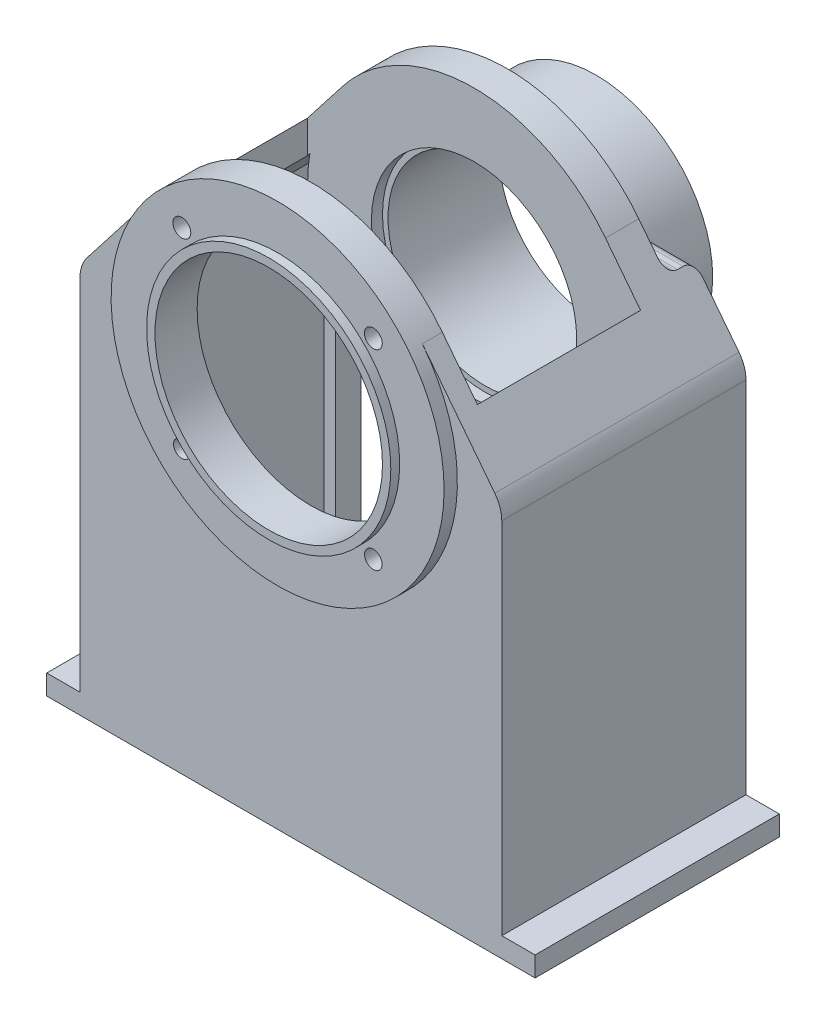
SolidWorks part; units mm, degrees
ref_plane "Front Plane" through (0, 0, 0) normal (0, 0, 1) x (1, 0, 0)
ref_plane "Top Plane" through (0, 0, 0) normal (0, 1, 0) x (1, 0, 0)
ref_plane "Right Plane" through (0, 0, 0) normal (1, 0, 0) x (0, 0, -1)
ref_plane "Plane1" through (0, 0, -1277.693) normal (0, 0, 1) x (1, 0, 0)
sketch "Sketch1" plane through (0, 0, -1277.693) normal (0, 0, 1) x (1, 0, 0)
  line L0 (671.2306, 234.744) -> (711.2306, 234.744)
  line L1 (711.2306, 234.744) -> (521.2306, 479.1294)
  line L2 (521.2306, 479.1294) -> (331.2306, 234.744)
  line L3 (331.2306, 234.744) -> (371.2306, 234.744)
  arc A0 (371.2306, 234.744) -> (671.2306, 234.744) centre (521.2306, 234.744) ccw
  dimension "D1" = 150
  dimension "D2" = 190
  dimension "D3" = 380
  dimension "D4" = 244.3855
extrude "Boss-Extrude1" add sketch "Sketch1" against normal blind 7
sketch "Sketch2" plane through (0, 234.744, 0) normal (0, -1, 0) x (1, 0, 0)
  line L0 (741.2306, -1284.693) -> (693.2306, -1284.693)
  line L1 (693.2306, -1284.693) -> (693.2306, -1277.693)
  line L2 (693.2306, -1277.693) -> (741.2306, -1277.693)
  line L3 (741.2306, -1277.693) -> (741.2306, -1284.693)
  line L4 (671.2306, -1284.693) -> (671.2306, -1277.693) construction
  line L5 (671.2306, -1277.693) -> (711.2306, -1277.693) construction
  dimension "D1" = 22
  dimension "D2" = 70
  dimension "D3" = 7
extrude "Boss-Extrude2" add sketch "Sketch2" along normal blind 352
sketch "Sketch3" plane through (0, 234.744, 0) normal (0, -1, 0) x (1, 0, 0)
  line L0 (349.2306, -1284.693) -> (331.2306, -1284.693)
  line L1 (331.2306, -1284.693) -> (331.2306, -1277.693)
  line L2 (331.2306, -1277.693) -> (349.2306, -1277.693)
  line L3 (349.2306, -1277.693) -> (349.2306, -1284.693)
  line L4 (331.2306, -1284.693) -> (331.2306, -1277.693) construction
  line L5 (331.2306, -1277.693) -> (371.2306, -1277.693) construction
  dimension "D1" = 18
  dimension "D2" = 7
extrude "Boss-Extrude3" add sketch "Sketch3" along normal blind 352
sketch "Sketch4" plane through (0, 0, -1284.693) normal (0, 0, -1) x (-1, 0, 0)
  line L0 (-331.2306, -117.256) -> (-741.2306, -117.256)
  line L1 (-741.2306, -117.256) -> (-741.2306, 234.744)
  line L2 (-741.2306, 234.744) -> (-711.2306, 234.744)
  line L3 (-711.2306, 234.744) -> (-521.2306, 479.1294)
  line L4 (-521.2306, 479.1294) -> (-331.2306, 234.744)
  line L5 (-331.2306, 234.744) -> (-331.2306, -117.256)
  line L6 (-331.2306, -117.256) -> (-331.2306, 234.744) construction
  line L7 (-331.2306, -117.256) -> (-349.2306, -117.256) construction
  dimension "D1" = 190
  dimension "D2" = 380
  dimension "D3" = 410
  dimension "D4" = 352
  dimension "D5" = 596.3855
extrude "Boss-Extrude4" add sketch "Sketch4" along normal blind 18
sketch "Sketch5" plane through (0, 0, -1277.693) normal (0, 0, 1) x (1, 0, 0)
  line L0 (371.2306, 234.744) -> (354.0306, 234.744)
  line L1 (354.0306, 234.744) -> (349.2306, 228.57)
  line L2 (349.2306, 228.57) -> (349.2306, -117.256)
  line L3 (349.2306, -117.256) -> (331.2306, -117.256)
  line L4 (331.2306, -117.256) -> (331.2306, 234.744)
  line L5 (331.2306, 234.744) -> (521.2306, 479.1294)
  line L6 (521.2306, 479.1294) -> (711.2306, 234.744)
  line L7 (711.2306, 234.744) -> (741.2306, 234.744)
  line L8 (741.2306, 234.744) -> (741.2306, -117.256)
  line L9 (741.2306, -117.256) -> (693.2306, -117.256)
  line L10 (693.2306, -117.256) -> (693.2306, 228.57)
  line L11 (693.2306, 228.57) -> (688.4306, 234.744)
  line L12 (688.4306, 234.744) -> (671.2306, 234.744)
  line L13 (741.2306, -117.256) -> (741.2306, 234.744) construction
  line L14 (741.2306, -117.256) -> (693.2306, -117.256) construction
  arc A0 (671.2306, 234.744) -> (371.2306, 234.744) centre (521.2306, 234.744) cw
  dimension "D1" = 150
  dimension "D2" = 30
  dimension "D3" = 48
  dimension "D4" = 52.8
  dimension "D5" = 220
  dimension "D6" = 387.2
  dimension "D7" = 392
  dimension "D8" = 410
  dimension "D9" = 345.8261
  dimension "D10" = 352
  dimension "D11" = 596.3855
extrude "Boss-Extrude5" add sketch "Sketch5" along normal blind 30
sketch "Sketch6" plane through (0, 0, -1247.693) normal (0, 0, 1) x (1, 0, 0)
  line L0 (371.2306, 256.8673) -> (349.2306, 228.57)
  line L1 (349.2306, 228.57) -> (349.2306, -117.256)
  line L2 (349.2306, -117.256) -> (331.2306, -117.256)
  line L3 (331.2306, -117.256) -> (331.2306, 234.744)
  line L4 (331.2306, 234.744) -> (371.2306, 286.1935)
  line L5 (371.2306, 286.1935) -> (371.2306, 256.8673)
  line L6 (741.2306, -117.256) -> (741.2306, 234.744) construction
  line L7 (693.2306, -117.256) -> (741.2306, -117.256) construction
  dimension "D1" = 370
  dimension "D2" = 392
  dimension "D3" = 410
  dimension "D4" = 345.8261
  dimension "D5" = 352
  dimension "D6" = 374.1233
  dimension "D7" = 403.4496
extrude "Boss-Extrude6" add sketch "Sketch6" along normal blind 147
sketch "Sketch7" plane through (0, 0, -1247.693) normal (0, 0, 1) x (1, 0, 0)
  line L0 (741.2306, -117.256) -> (693.2306, -117.256)
  line L1 (693.2306, -117.256) -> (693.2306, 228.57)
  line L2 (693.2306, 228.57) -> (671.2306, 256.8673)
  line L3 (671.2306, 256.8673) -> (671.2306, 286.1935)
  line L4 (671.2306, 286.1935) -> (711.2306, 234.744)
  line L5 (711.2306, 234.744) -> (741.2306, 234.744)
  line L6 (741.2306, 234.744) -> (741.2306, -117.256)
  line L7 (371.2306, 256.8673) -> (371.2306, 286.1935) construction
  line L8 (354.0306, 234.744) -> (371.2306, 234.744) construction
  dimension "D1" = 300
  dimension "D2" = 322
  dimension "D3" = 340
  dimension "D4" = 370
  dimension "D5" = 22.1233
  dimension "D6" = 51.4496
  dimension "D7" = 6.1739
  dimension "D8" = 352
extrude "Boss-Extrude7" add sketch "Sketch7" along normal blind 147
sketch "Sketch8" plane through (0, 0, -1100.693) normal (0, 0, 1) x (1, 0, 0)
  line L0 (331.2306, -117.256) -> (331.2306, 234.744)
  line L1 (331.2306, 234.744) -> (402.8096, 326.8116)
  line L2 (639.6517, 326.8116) -> (711.2306, 234.744)
  line L3 (711.2306, 234.744) -> (741.2306, 234.744)
  line L4 (741.2306, 234.744) -> (741.2306, -117.256)
  line L5 (741.2306, -117.256) -> (331.2306, -117.256)
  line L6 (331.2306, 234.744) -> (331.2306, -117.256) construction
  arc A0 (402.8096, 326.8116) -> (639.6517, 326.8116) centre (521.2306, 234.744) cw
  dimension "D1" = 150
  dimension "D2" = 71.5789
  dimension "D3" = 190
  dimension "D4" = 352
  dimension "D6" = 410
extrude "Boss-Extrude8" add sketch "Sketch8" along normal blind 18
sketch "Sketch9" plane through (0, 234.744, 0) normal (0, 1, 0) x (-1, 0, 0)
  line L0 (-711.2306, -1302.693) -> (-711.2306, -1082.693)
  line L1 (-711.2306, -1082.693) -> (-741.2306, -1082.693)
  line L2 (-741.2306, -1082.693) -> (-741.2306, -1302.693)
  line L3 (-741.2306, -1302.693) -> (-711.2306, -1302.693)
  line L4 (-741.2306, -1302.693) -> (-741.2306, -1082.693) construction
  dimension "D1" = 30
  dimension "D2" = 220
extrude "Cut-Extrude1" cut sketch "Sketch9" against normal blind 334
sketch "Sketch10" plane through (0, 0, -1247.693) normal (0, 0, 1) x (1, 0, 0)
  line L0 (671.2306, 234.744) -> (688.4306, 234.744)
  line L1 (688.4306, 234.744) -> (669.1709, 259.5166)
  line L2 (671.2306, 286.1935) -> (671.2306, 256.8673) construction
  arc A0 (669.1709, 259.5166) -> (671.2306, 234.744) centre (521.2306, 234.744) cw
  dimension "D1" = 150
  dimension "D2" = 17.2
  dimension "D3" = 2.0598
  dimension "D4" = 150
extrude "Cut-Extrude2" cut sketch "Sketch10" against normal blind 30
sketch "Sketch11" plane through (0, 0, -1247.693) normal (0, 0, 1) x (1, 0, 0)
  line L0 (373.2904, 259.5166) -> (354.0306, 234.744)
  line L1 (354.0306, 234.744) -> (371.2306, 234.744)
  line L2 (671.2306, 286.1935) -> (671.2306, 256.8673) construction
  arc A0 (371.2306, 234.744) -> (373.2904, 259.5166) centre (521.2306, 234.744) cw
  dimension "D1" = 150
  dimension "D2" = 150
  dimension "D3" = 297.9402
  dimension "D4" = 219.6128
  dimension "D5" = 317.2
extrude "Cut-Extrude3" cut sketch "Sketch11" against normal blind 30
sketch "Sketch12" plane through (331.2306, 0, 0) normal (-1, 0, 0) x (0, 0, 1)
  line L0 (-1082.693, -99.256) -> (-1082.693, -117.256)
  line L1 (-1082.693, -117.256) -> (-1302.693, -117.256)
  line L2 (-1302.693, -117.256) -> (-1302.693, -99.256)
  line L3 (-1302.693, -99.256) -> (-1082.693, -99.256)
  line L4 (-1302.693, 234.744) -> (-1082.693, 234.744) construction
  line L5 (-1302.693, -117.256) -> (-1302.693, 234.744) construction
  dimension "D1" = 220
  dimension "D2" = 334
  dimension "D3" = 352
extrude "Boss-Extrude9" add sketch "Sketch12" along normal blind 30
sketch "Sketch13" plane through (0, 0, -1082.693) normal (0, 0, 1) x (1, 0, 0)
  line L0 (711.2306, -99.256) -> (711.2306, 234.744) construction
  line L1 (711.2306, -99.256) -> (741.2306, -99.256) construction
  circle A0 centre (521.2306, 234.744) radius 150
  dimension "D1" = 300
  dimension "D2" = 190
  dimension "D3" = 334
extrude "Boss-Extrude10" add sketch "Sketch13" along normal blind 12
sketch "Sketch14" plane through (0, 0, -1247.693) normal (0, 0, 1) x (1, 0, 0)
  line L0 (412.8196, 184.744) -> (379.8093, 184.744)
  line L1 (662.652, 184.744) -> (629.6417, 184.744)
  line L2 (671.2306, 286.1935) -> (671.2306, 256.8673) construction
  arc A0 (629.6417, 184.744) -> (412.8196, 184.744) centre (521.2306, 234.744) cw
  arc A1 (379.8093, 184.744) -> (662.652, 184.744) centre (521.2306, 234.744) ccw
  dimension "D1" = 119.3857
  dimension "D2" = 150
  dimension "D3" = 8.5786
  dimension "D4" = 41.5889
  dimension "D5" = 51.4496
extrude "Cut-Extrude4" cut sketch "Sketch14" against normal blind 37
sketch "Sketch15" plane through (0, 0, -1302.693) normal (0, 0, -1) x (-1, 0, 0)
  line L0 (-351.2306, -117.256) -> (-691.2306, -117.256)
  line L1 (-691.2306, -117.256) -> (-691.2306, 123.3582)
  line L2 (-691.2306, 123.3582) -> (-351.2306, 123.3582)
  line L3 (-351.2306, 123.3582) -> (-351.2306, -117.256)
  line L4 (-741.2306, -99.256) -> (-741.2306, -117.256) construction
  line L5 (-741.2306, -117.256) -> (-301.2306, -117.256) construction
  dimension "D1" = 50
  dimension "D2" = 390
  dimension "D3" = 240.6143
extrude "Boss-Extrude11" add sketch "Sketch15" along normal blind 5
sketch "Sketch16" plane through (0, 0, -1307.693) normal (0, 0, -1) x (-1, 0, 0)
  line L0 (-359.2306, -117.256) -> (-359.2306, 115.3582)
  line L1 (-359.2306, 115.3582) -> (-683.2306, 115.3582)
  line L2 (-683.2306, 115.3582) -> (-683.2306, -117.256)
  line L3 (-683.2306, -117.256) -> (-359.2306, -117.256)
  line L4 (-351.2306, -117.256) -> (-351.2306, 123.3582) construction
  line L5 (-351.2306, 123.3582) -> (-691.2306, 123.3582) construction
  dimension "D1" = 8
  dimension "D2" = 332
  dimension "D3" = 8
  dimension "D4" = 240.6143
extrude "Cut-Extrude5" cut sketch "Sketch16" against normal up to next
sketch "Sketch17" plane through (0, 0, -1302.693) normal (0, 0, -1) x (-1, 0, 0)
  line L0 (-521.2306, 479.1294) -> (-664.583, 294.744)
  line L1 (-664.583, 294.744) -> (-377.8783, 294.744)
  line L2 (-377.8783, 294.744) -> (-521.2306, 479.1294)
  line L3 (-301.2306, -99.256) -> (-301.2306, -117.256) construction
  line L4 (-351.2306, -117.256) -> (-301.2306, -117.256) construction
  dimension "D1" = 76.6476
  dimension "D2" = 220
  dimension "D3" = 363.3524
  dimension "D4" = 412
  dimension "D5" = 596.3855
extrude "Cut-Extrude6" cut sketch "Sketch17" against normal blind 25
sketch "Sketch18" plane through (0, 0, -1070.693) normal (0, 0, 1) x (1, 0, 0)
  circle A0 centre (521.2306, 234.744) radius 110
  dimension "D1" = 220
extrude "Boss-Extrude12" add sketch "Sketch18" along normal blind 8
ref_plane "Plane2" through (280.2795, 402.5208, 0) normal (0.5714, 0.8207, 0) x (-0.8207, 0.5714, 0)
sketch "Sketch19" plane through (280.2795, 402.5208, 0) normal (0.5714, 0.8207, 0) x (-0.8207, 0.5714, 0)
  line L0 (-188.6095, -1277.693) -> (-293.6095, -1277.693)
  line L1 (-293.6095, -1277.693) -> (-293.6095, -1357.693)
  line L2 (-293.6095, -1357.693) -> (-188.6095, -1357.693)
  line L3 (-188.6095, -1357.693) -> (-188.6095, -1277.693)
  line L4 (-293.6095, -1277.693) -> (-293.6095, -1357.693) construction
  dimension "D1" = 105
  dimension "D2" = 80
revolve "Revolve1" add sketch "Sketch19" angle 360 about L4
hole_wizard "Hole1" positions "Sketch21" profile "Sketch20" legacy
sketch "Sketch21" plane through (0, 0, -1062.693) normal (0, 0, 1) x (1, 0, 0)
  point P0 (521.2306, 234.744)
sketch "Sketch20" plane through (521.2306, 234.744, -1062.693) normal (1, 0, 0) x (0, -1, 0)
  line L0 (0, 0) -> (0, 38)
  line L1 (0, 38) -> (102.5, 38)
  line L2 (102.5, 38) -> (102.5, 0)
  line L3 (102.5, 0) -> (0, 0)
  line L4 (0, 110) -> (0, -10) construction
  dimension "直径" = 205
  dimension "深度" = 38
hole_wizard "M10 counterbore hole1" positions "Sketch23" profile "Sketch22" counterbore size "M10" standard "ANSI Metric"
sketch "Sketch23" plane through (0, 0, -1357.693) normal (0, 0, -1) x (-1, 0, 0)
  point P0 (-614.8306, 234.744)
  point P1 (-521.2306, 141.144)
  point P2 (-427.6306, 234.744)
  point P3 (-521.2306, 328.344)
sketch "Sketch22" plane through (614.8306, 234.744, -1357.693) normal (1, 0, 0) x (0, 1, 0)
  line L0 (0, 0) -> (0, 45)
  line L1 (0, 45) -> (6, 45)
  line L2 (6, 45) -> (6, 12)
  line L3 (6, 12) -> (9, 12)
  line L4 (9, 12) -> (9, 0)
  line L5 (9, 0) -> (0, 0)
  line L10 (0, 45) -> (-6, 45) construction
  line L11 (0, -6.35) -> (0, 107.95) construction
  dimension "孔直径" = 12
  dimension "孔深度" = 45
  dimension "柱形沉头孔直径" = 18
  dimension "柱形沉头孔深度" = 12
  dimension "导头角度" = 180
hole_wizard "Hole2" positions "Sketch25" profile "Sketch24" legacy
sketch "Sketch25" plane through (0, 0, -1247.693) normal (0, 0, 1) x (1, 0, 0)
  point P0 (521.2306, 234.744)
sketch "Sketch24" plane through (521.2306, 234.744, -1247.693) normal (1, 0, 0) x (0, -1, 0)
  line L0 (0, 0) -> (0, 110)
  line L1 (0, 110) -> (87.5, 110)
  line L2 (87.5, 110) -> (87.5, 10)
  line L3 (87.5, 10) -> (92.5, 10)
  line L4 (92.5, 10) -> (92.5, 0)
  line L5 (92.5, 0) -> (0, 0)
  line L6 (0, 110) -> (0, -10) construction
  dimension "直径" = 175
  dimension "深度" = 110
  dimension "柱坑直径" = 185
  dimension "柱坑深度" = 10
fillet "Fillet1" radius 10 6 edges at (683.2306, 115.3582, -1296.193) (359.2306, 115.3582, -1296.193) (635.9911, 294.744, -1277.693) (406.4702, 294.744, -1277.693) (406.4702, 294.744, -1302.693) (635.9911, 294.744, -1302.693)
fillet "Fillet2" radius 18 2 edges at (691.2306, 123.3582, -1305.193) (351.2306, 123.3582, -1305.193)
fillet "Fillet3" radius 30 2 edges at (711.2306, 234.744, -1192.693) (331.2306, 234.744, -1192.693)
fillet "Fillet4" radius 150 1 edges at (521.2306, 479.1294, -1262.693)
sketch "Sketch26" plane through (0, 0, -1070.693) normal (0, 0, 1) x (1, 0, 0)
  circle A0 centre (434.9636, 321.011) radius 8.055
  circle A1 centre (607.4977, 321.011) radius 8.055
  circle A2 centre (607.4977, 148.4769) radius 7.9277
  circle A3 centre (434.9636, 148.4769) radius 7.5096
extrude "Cut-Extrude8" cut sketch "Sketch26" against normal blind 41
